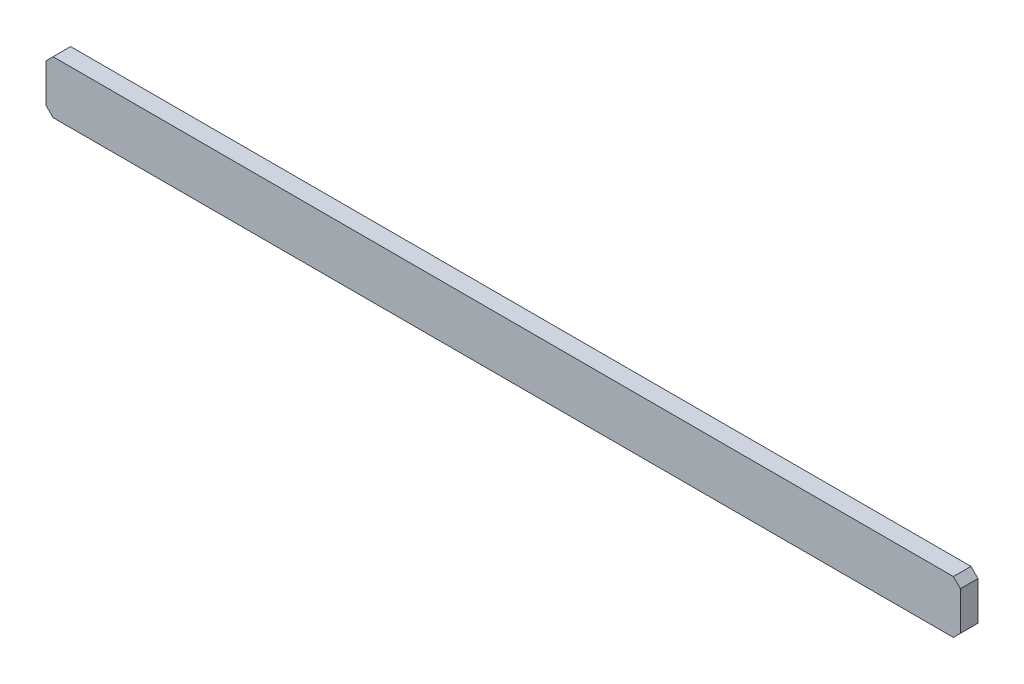
SolidWorks part; units mm, degrees
ref_plane "前视基准面" through (0, 0, 0) normal (0, 0, 1) x (1, 0, 0)
ref_plane "上视基准面" through (0, 0, 0) normal (0, 1, 0) x (1, 0, 0)
ref_plane "右视基准面" through (0, 0, 0) normal (1, 0, 0) x (0, 0, -1)
sketch "草图1" plane through (0, 0, 0) normal (0, 0, 1) x (1, 0, 0)
  line L1 (-130, -7.5) -> (130, -7.5)
  line L2 (-130, -7.5) -> (-130, 7.5)
  line L3 (-130, 7.5) -> (130, 7.5)
  line L4 (130, -7.5) -> (130, 7.5)
  line L5 (-130, -7.5) -> (130, 7.5) construction
  line L6 (-130, 7.5) -> (130, -7.5) construction
  point P0 (0, 0)
  dimension "D1" = 260
  dimension "D2" = 15
extrude "凸台-拉伸1" add sketch "草图1" along normal blind 5
chamfer "倒角1" distance 2 angle 45 4 edges at (130, -7.5, 2.5) (130, 7.5, 2.5) (-130, -7.5, 2.5) (-130, 7.5, 2.5)
